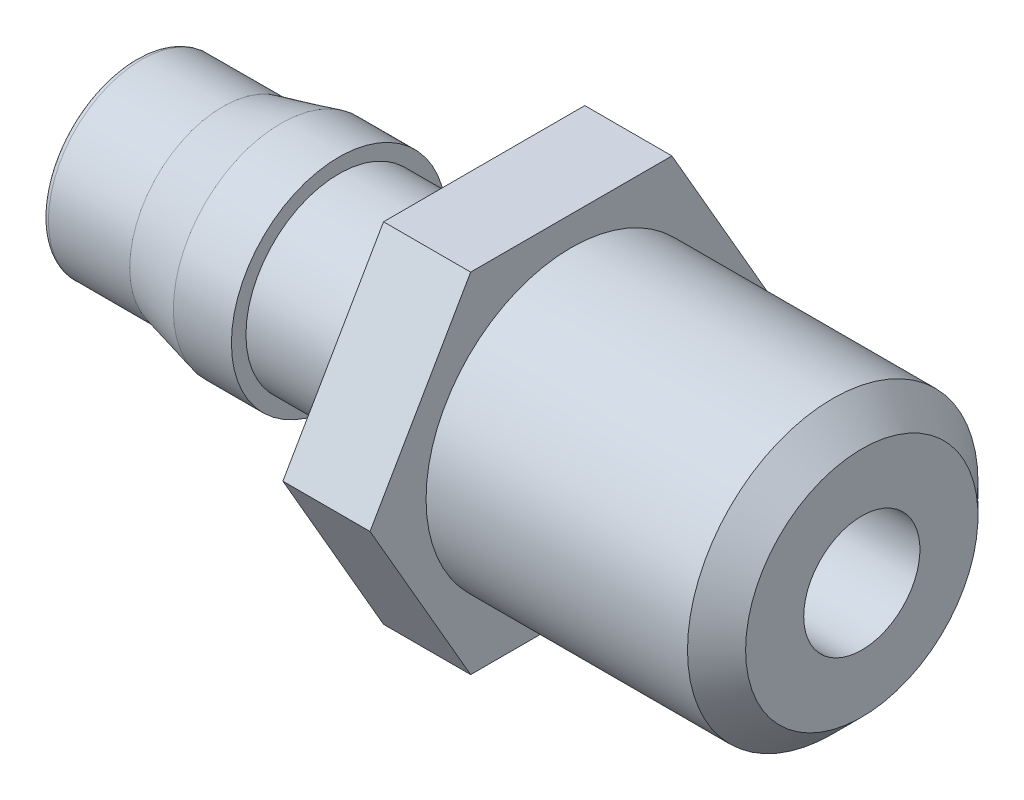
SolidWorks part; units mm, degrees
material "H62"
ref_plane "Front Plane" through (0, 0, 0) normal (0, 0, 1) x (1, 0, 0)
ref_plane "Top Plane" through (0, 0, 0) normal (0, 1, 0) x (1, 0, 0)
ref_plane "Right Plane" through (0, 0, 0) normal (1, 0, 0) x (0, 0, -1)
sketch "Sketch1" plane through (0, 0, 0) normal (0, 0, 1) x (1, 0, 0)
  line L0 (0, 0) -> (22.0497, 0) construction
  line L1 (0, 1) -> (12.5, 1)
  line L2 (0, 1) -> (0, 1.6)
  line L3 (0, 1.6) -> (1.5, 1.6)
  line L4 (1.5, 1.6) -> (2.5, 1.85)
  line L5 (2.5, 1.85) -> (3.5, 1.85)
  line L6 (3.5, 1.85) -> (3.5, 1.6)
  line L7 (3.5, 1.6) -> (6, 1.6)
  line L8 (6, 1.6) -> (6, 4.5)
  line L9 (6, 4.5) -> (7.5, 4.5)
  line L10 (7.5, 4.5) -> (7.5, 2.5)
  line L11 (7.5, 2.5) -> (12.5, 2.5)
  line L12 (12.5, 2.5) -> (12.5, 1)
  dimension "D1" = 12.5
  dimension "D2" = 1.5
  dimension "D3" = 1
  dimension "D4" = 2
  dimension "D5" = 3.2
  dimension "D6" = 3.7
  dimension "D7" = 3.2
  dimension "D8" = 9
  dimension "D9" = 5
  dimension "D10" = 2.5
  dimension "D11" = 5
  dimension "D12" = 6
revolve "Revolve1" add sketch "Sketch1" angle 360 about L0
cosmetic thread "Cosmetic Thread1" parameters "D1"=5, "D2"=4.85
sketch "Sketch2" plane through (7.5, 0, 0) normal (1, 0, 0) x (0, 0, -1)
  line L1 (1.7321, -3) -> (3.4641, 0)
  line L2 (3.4641, 0) -> (1.7321, 3)
  line L3 (1.7321, 3) -> (-1.7321, 3)
  line L4 (-1.7321, 3) -> (-3.4641, 0)
  line L5 (-3.4641, 0) -> (-1.7321, -3)
  line L6 (-1.7321, -3) -> (1.7321, -3)
  circle A0 centre (0, 0) radius 3 construction
  dimension "D1" = 6
extrude "Cut-Extrude3" cut sketch "Sketch2" against normal blind 10 flip side to cut
fillet "Fillet1" radius 0.1 1 edges at (0, 0, 1.6)
chamfer "Chamfer1" distance 0.5 angle 45 1 edges at (12.5, 0, 2.5)
